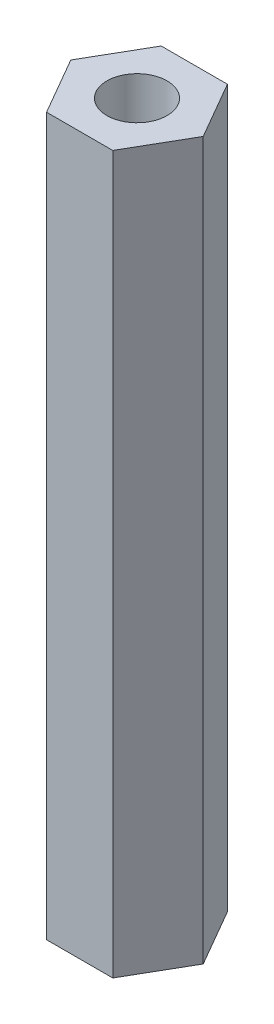
from build123d import *

# Parameters (mm, degrees)
BOSS_EXTRUDE1_DEPTH = 63.5
SKETCH2_R           = 2.667
CUT_EXTRUDE1_DEPTH  = 127
SCALE1_SCALE        = 2


with BuildPart() as part:
    # Sketch1 → Boss-Extrude1 (new body)
    with BuildSketch(Plane(origin=(0, 0, 0), x_dir=(1, 0, 0), z_dir=(0, 1, 0))):
        Polygon((2.932939367, -5.08), (5.865878735, 0), (2.932939367, 5.08), (-2.932939367, 5.08), (-5.865878735, 0), (-2.932939367, -5.08), align=None)
    extrude(amount=BOSS_EXTRUDE1_DEPTH)

    # Sketch2 → Cut-Extrude1 (cut)
    with BuildSketch(Plane(origin=(0, 0, 0), x_dir=(1, 0, 0), z_dir=(0, 1, 0))):
        with Locations(Location((0, 0, 0), (0, 0, 270))):
            Circle(SKETCH2_R)
    extrude(amount=CUT_EXTRUDE1_DEPTH, mode=Mode.SUBTRACT)


with BuildPart() as part_1:
    # Scale1: scaled about (0, 0, 0)
    add(part.part.scale(SCALE1_SCALE))


solid = part_1.part
